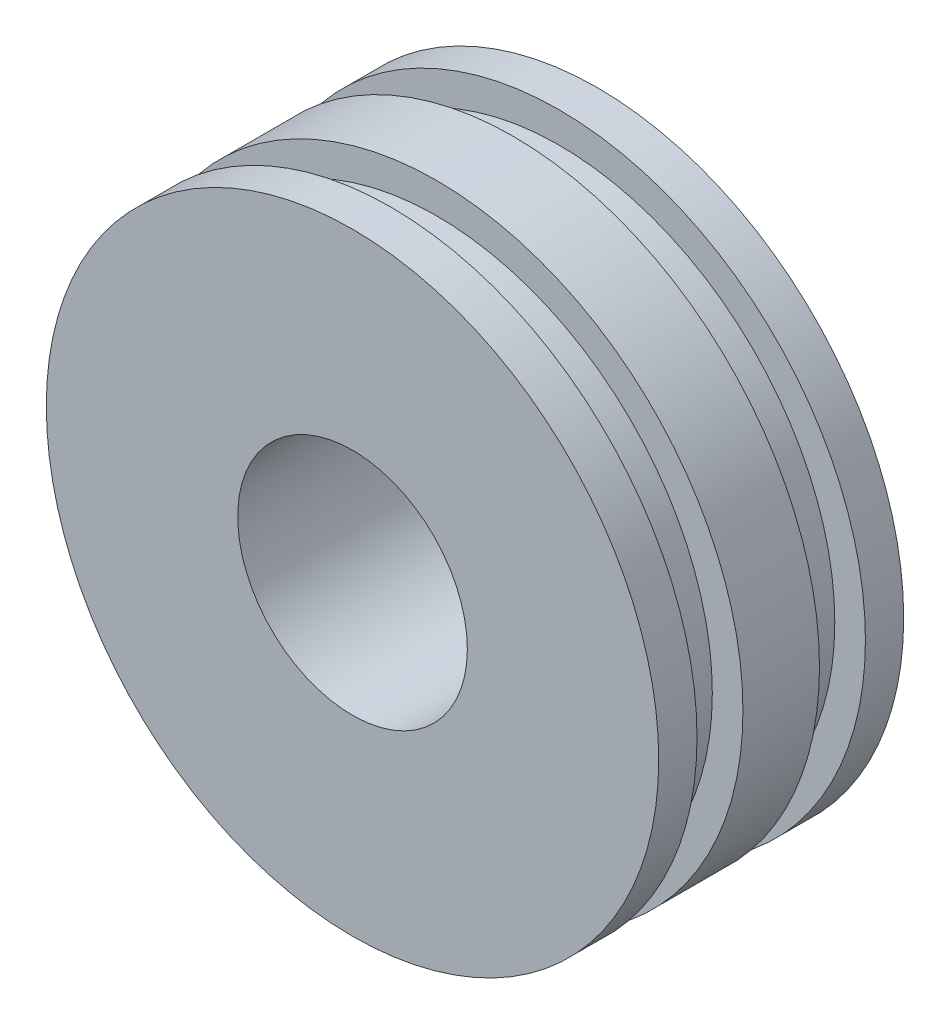
from build123d import *

# Parameters (mm, degrees)
SKETCH_1_R          = 100
SKETCH_1_R_2        = 37.5
EXTRUDE_1_DEPTH     = 40
SKETCH_2_R          = 100
SKETCH_2_R_2        = 90
CUT_EXTRUDE_1_DEPTH = 7.5


with BuildPart() as part:
    # 草图1 → 凸台-拉伸1 (new, symmetric)
    with BuildSketch(Plane.XY):
        Circle(SKETCH_1_R)
        Circle(SKETCH_1_R_2, mode=Mode.SUBTRACT)
    extrude(amount=EXTRUDE_1_DEPTH, both=True)

    # 草图2 → 切除-拉伸1 (cut, symmetric)
    with BuildSketch(Plane.XY.offset(20)):
        Circle(SKETCH_2_R)
        Circle(SKETCH_2_R_2, mode=Mode.SUBTRACT)
    cut_extrude_1 = extrude(amount=CUT_EXTRUDE_1_DEPTH, both=True, mode=Mode.SUBTRACT)

    # 镜向1: 切除-拉伸1 across plane
    add(cut_extrude_1.mirror(Plane.XY), mode=Mode.SUBTRACT)


solid = part.part
